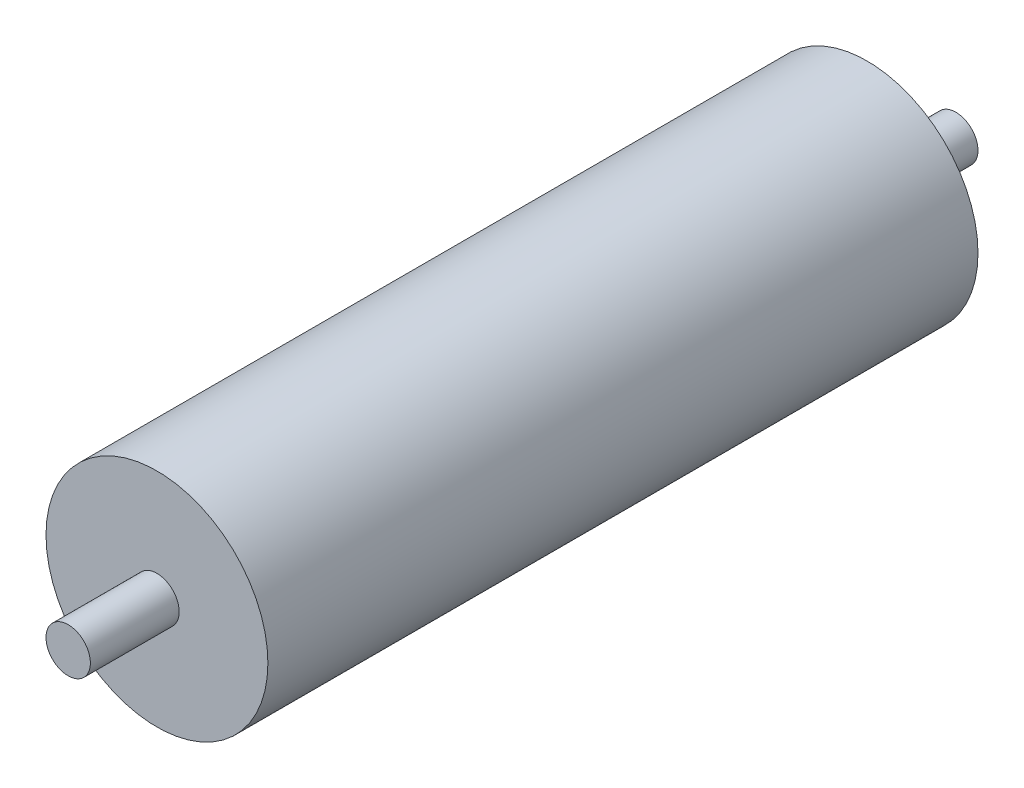
SolidWorks part; units mm, degrees
ref_plane "Front Plane" through (0, 0, 0) normal (0, 0, 1) x (1, 0, 0)
ref_plane "Top Plane" through (0, 0, 0) normal (0, 1, 0) x (1, 0, 0)
ref_plane "Right Plane" through (0, 0, 0) normal (1, 0, 0) x (0, 0, -1)
other "Configuration Table"
sketch "Sketch1" plane through (0, 0, 0) normal (0, 0, 1) x (1, 0, 0)
  line L0 (0, 70.7496) -> (0, -70.7496) construction
  circle A0 centre (0, 0) radius 25
  point P4 (0, 0)
  dimension "D1" = 50
extrude "Boss-Extrude1" add sketch "Sketch1" along normal blind 160
sketch "Sketch2" plane through (0, 0, 0) normal (0, 0, -1) x (-1, 0, 0)
  circle A0 centre (0, 0) radius 5
  dimension "D1" = 10
extrude "Boss-Extrude2" add sketch "Sketch2" along normal blind 20
ref_plane "Plane1" through (0, 0, 80) normal (0, 0, -1) x (-1, 0, 0)
mirror "Mirror1" about plane through (0, 0, 80) normal (0, 0, -1) of "Boss-Extrude2"
